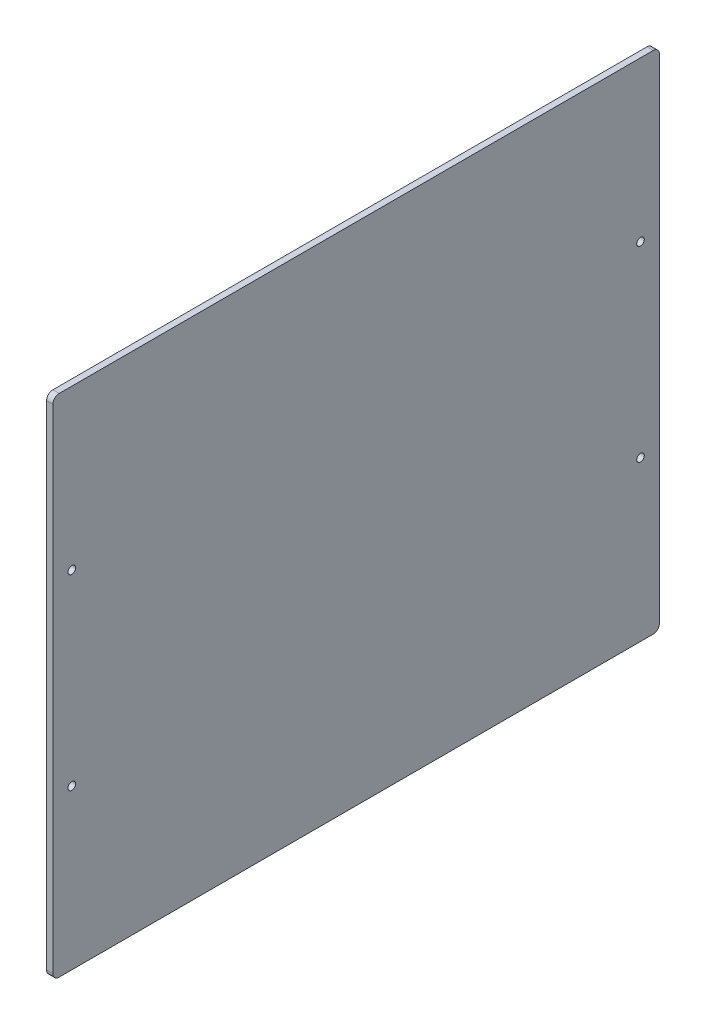
from build123d import *

# Parameters (mm, degrees)
SKETCH_1_W          = 480
SKETCH_1_H          = 400
EXTRUDE_1_DEPTH     = 5
SKETCH_2_R          = 3
CUT_EXTRUDE_1_DEPTH = 313.449995999
FILLET_1_R          = 5


with BuildPart() as part:
    # 草图1 → 凸台-拉伸1 (new body)
    with BuildSketch(Plane(origin=(0, 0, 0), x_dir=(0, 0, -1), z_dir=(1, 0, 0))):
        Rectangle(SKETCH_1_W, SKETCH_1_H)
    extrude(amount=EXTRUDE_1_DEPTH)

    # 草图2 → 切除-拉伸1 (cut, through all)
    with BuildSketch(Plane(origin=(5, 0, 0), x_dir=(0, 0, -1), z_dir=(1, 0, 0))):
        with Locations((-225, 74)):
            Circle(SKETCH_2_R)
        with Locations((225, 74)):
            Circle(SKETCH_2_R)
        with Locations((-225, -74)):
            Circle(SKETCH_2_R)
        with Locations((225, -74)):
            Circle(SKETCH_2_R)
    extrude(amount=-CUT_EXTRUDE_1_DEPTH, mode=Mode.SUBTRACT)

    # 圆角1
    fillet_1_edges = [part.edges().sort_by_distance(p)[0] for p in [
        (2.5, 200, 240),
        (2.5, 200, -240),
        (2.5, -200, -240),
        (2.5, -200, 240),
    ]]
    fillet(fillet_1_edges, radius=FILLET_1_R)


solid = part.part
